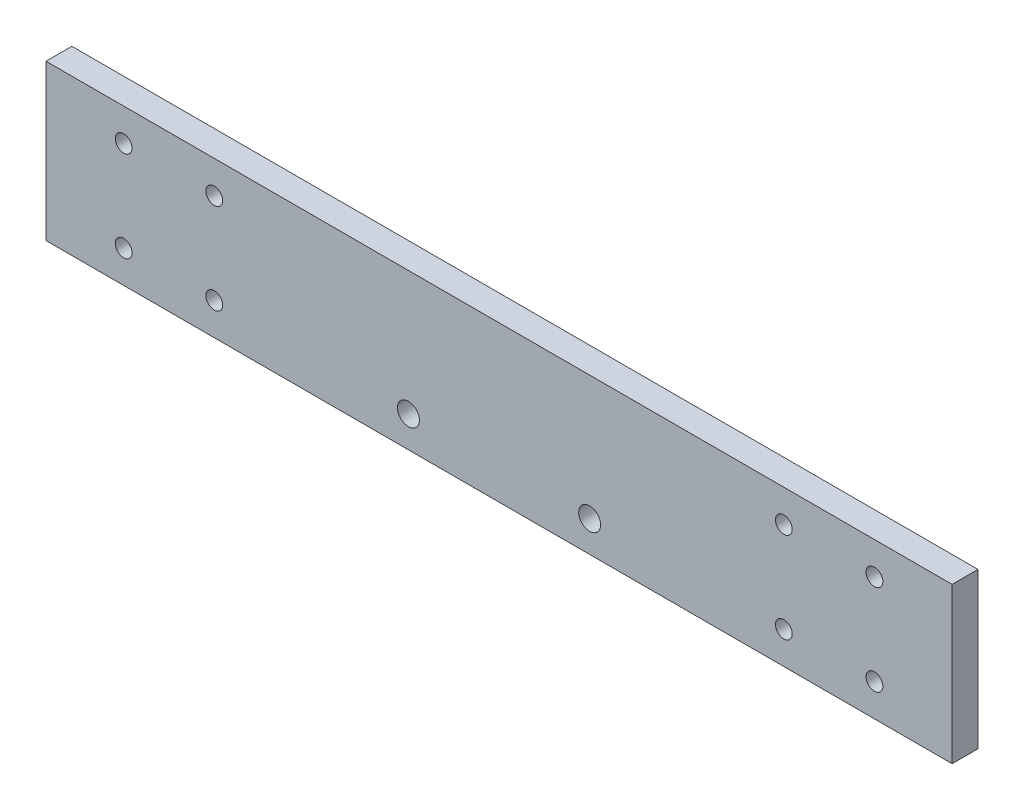
SolidWorks part; units mm, degrees
material "普通碳钢"
ref_plane "Front Plane" through (0, 0, 0) normal (0, 0, 1) x (1, 0, 0)
ref_plane "Top Plane" through (0, 0, 0) normal (0, 1, 0) x (1, 0, 0)
ref_plane "Right Plane" through (0, 0, 0) normal (1, 0, 0) x (0, 0, -1)
sketch "Sketch1" plane through (0, 0, 0) normal (0, 0, 1) x (1, 0, 0)
  line L0 (0, 0) -> (0, 60) construction
  line L1 (175, 0) -> (-175, 0)
  line L2 (175, 0) -> (175, 60)
  line L3 (175, 60) -> (-175, 60)
  line L4 (-175, 0) -> (-175, 60)
  line L7 (-175, 30) -> (175, 30) construction
  line L8 (-80, -265) -> (-80, 25) construction
  line L9 (-80, 25) -> (0, 25) construction
  circle A0 centre (-145, 47.5) radius 3.25
  circle A1 centre (-110, 47.5) radius 3.25
  circle A2 centre (-110, 12.5) radius 3.25
  circle A3 centre (-145, 12.5) radius 3.25
  circle A4 centre (110, 12.5) radius 3.25
  circle A5 centre (145, 12.5) radius 3.25
  circle A6 centre (110, 47.5) radius 3.25
  circle A7 centre (145, 47.5) radius 3.25
  dimension "D3" = 6.5
  dimension "D1" = 350
  dimension "D2" = 60
  dimension "D4" = 110
  dimension "D5" = 35
  dimension "D6" = 17.5
  dimension "D7" = 80
  dimension "D8" = 25
extrude "Boss-Extrude1" add sketch "Sketch1" along normal blind 10
hole_wizard "M10 Tapped Hole1" positions "Sketch2" profile "Sketch3" tap size "M10" standard "GB" end condition through all
sketch "Sketch2" plane through (0, 0, 10) normal (0, 0, 1) x (1, 0, 0)
  line L2 (-175, 0) -> (175, 0) construction
  line L3 (0, 0) -> (0, 60) construction
  line L4 (175, 60) -> (-175, 60) construction
  point P0 (-35, 12)
  point P21 (35, 12)
  dimension "D1" = 12
  dimension "D2" = 70
sketch "Sketch3" plane through (-35, 12, 10) normal (1, 0, 0) x (0, -1, 0)
  line L0 (0, 0) -> (0, 10)
  line L1 (0, 10) -> (4.25, 10)
  line L2 (4.25, 10) -> (4.25, 0)
  line L5 (4.25, 0) -> (0, 0)
  line L11 (0, -6.35) -> (0, 107.95) construction
  dimension "通孔螺纹孔钻头直径" = 8.5
  dimension "通孔螺纹孔钻头深度" = 10
cosmetic thread "Hole Cosmetic Thread1" parameters "D2"=10
cosmetic thread "Hole Cosmetic Thread2" parameters "D2"=10
